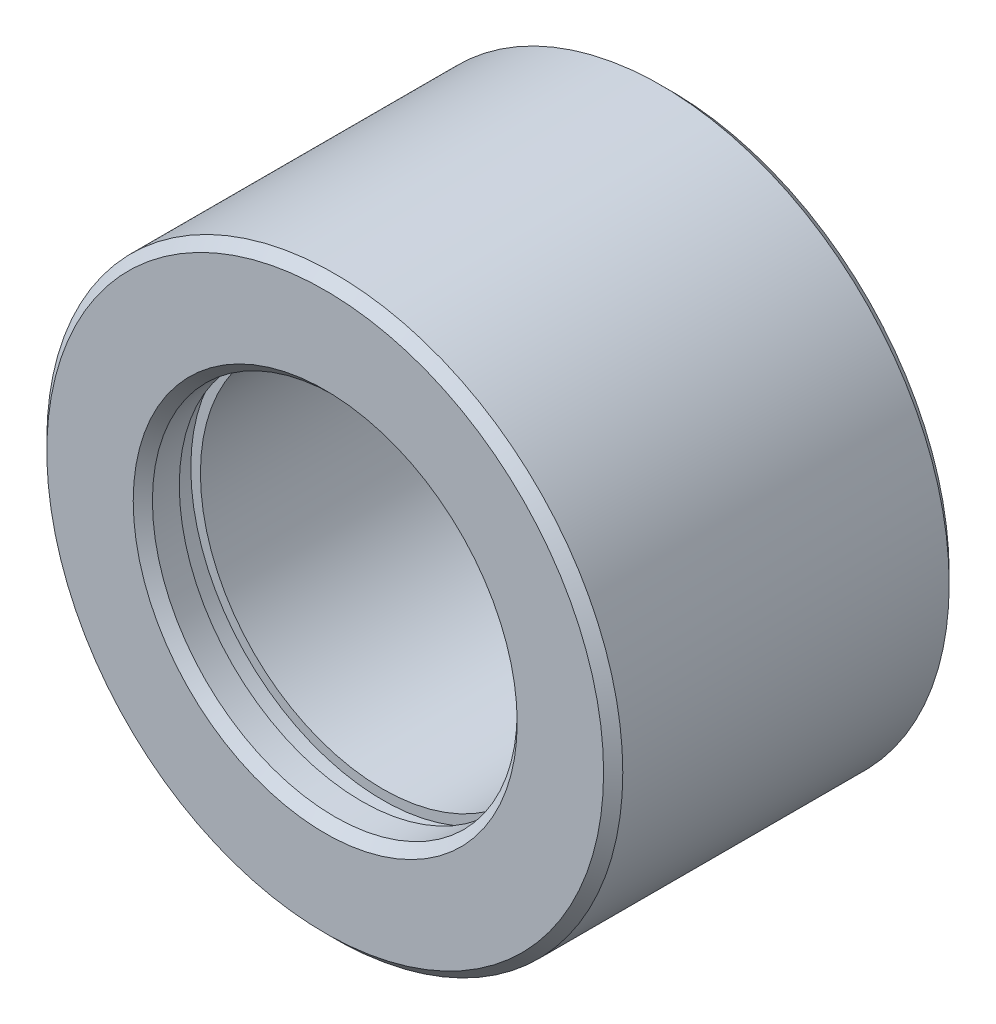
SolidWorks part; units mm, degrees
ref_plane "Front Plane" through (0, 0, 0) normal (0, 0, 1) x (1, 0, 0)
ref_plane "Top Plane" through (0, 0, 0) normal (0, 1, 0) x (1, 0, 0)
ref_plane "Right Plane" through (0, 0, 0) normal (1, 0, 0) x (0, 0, -1)
sketch "Sketch1" plane through (0, 0, 0) normal (0, 0, 1) x (1, 0, 0)
  circle A0 centre (0, 0) radius 15
  circle A1 centre (0, 0) radius 9.5
  dimension "D1" = 30
  dimension "D2" = 19
extrude "Boss-Extrude1" add sketch "Sketch1" along normal mid plane 18
sketch "Sketch2" plane through (0, 0, 0) normal (0, 0, 1) x (1, 0, 0)
  circle A0 centre (0, 0) radius 10
  circle A1 centre (0, 0) radius 9.5
  dimension "D1" = 20
extrude "Cut-Extrude1" cut sketch "Sketch2" along normal blind 1.1 from offset 6
mirror "Mirror1" about plane through (0, 0, 0) normal (0, 0, 1) of "Cut-Extrude1"
chamfer "Chamfer1" distance 0.5 angle 45 4 edges at (15, 0, -9) (15, 0, 9) (9.5, 0, -9) (9.5, 0, 9)
